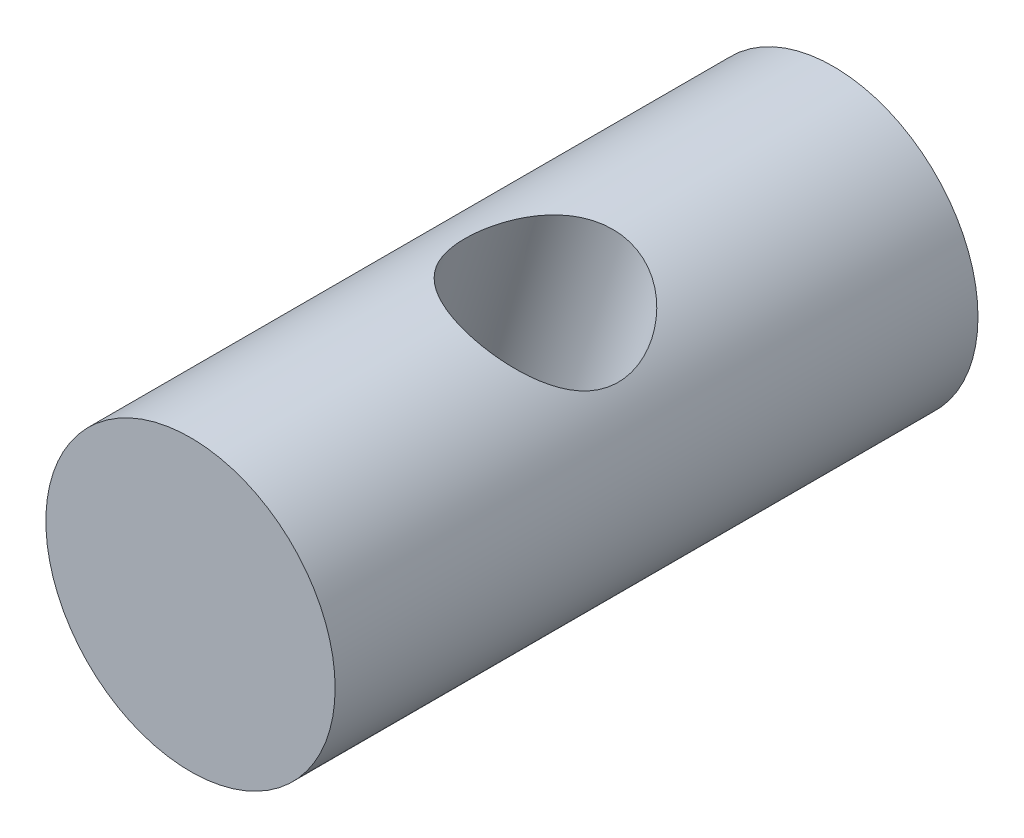
from build123d import *

# Parameters (mm, degrees)
SKETCH_1_R             = 4.5
EXTRUDE_1_DEPTH        = 20
HOLE_WIZARD_M6_1_D     = 5
HOLE_WIZARD_M6_1_DEPTH = 6
HOLE_WIZARD_M6_1_TIP   = 1.502151548


with BuildPart() as part:
    # 草图1 → 凸台-拉伸1 (new body)
    with BuildSketch(Plane.XY):
        Circle(SKETCH_1_R)
    extrude(amount=EXTRUDE_1_DEPTH)

    # M6 螺纹孔1
    with Locations(Plane(origin=(1.335069206, 4.297393421, 10.189708397), x_dir=(0.95497631577, -0.296682045829, 0), z_dir=(0.296682045829, 0.95497631577, 0))):
        with Locations((0, 0)):
            Hole(HOLE_WIZARD_M6_1_D / 2, depth=HOLE_WIZARD_M6_1_DEPTH)
            with Locations((0, 0, -(HOLE_WIZARD_M6_1_DEPTH + HOLE_WIZARD_M6_1_TIP / 2))):  # 118° drill point
                Cone(0, HOLE_WIZARD_M6_1_D / 2, HOLE_WIZARD_M6_1_TIP, mode=Mode.SUBTRACT)


solid = part.part
